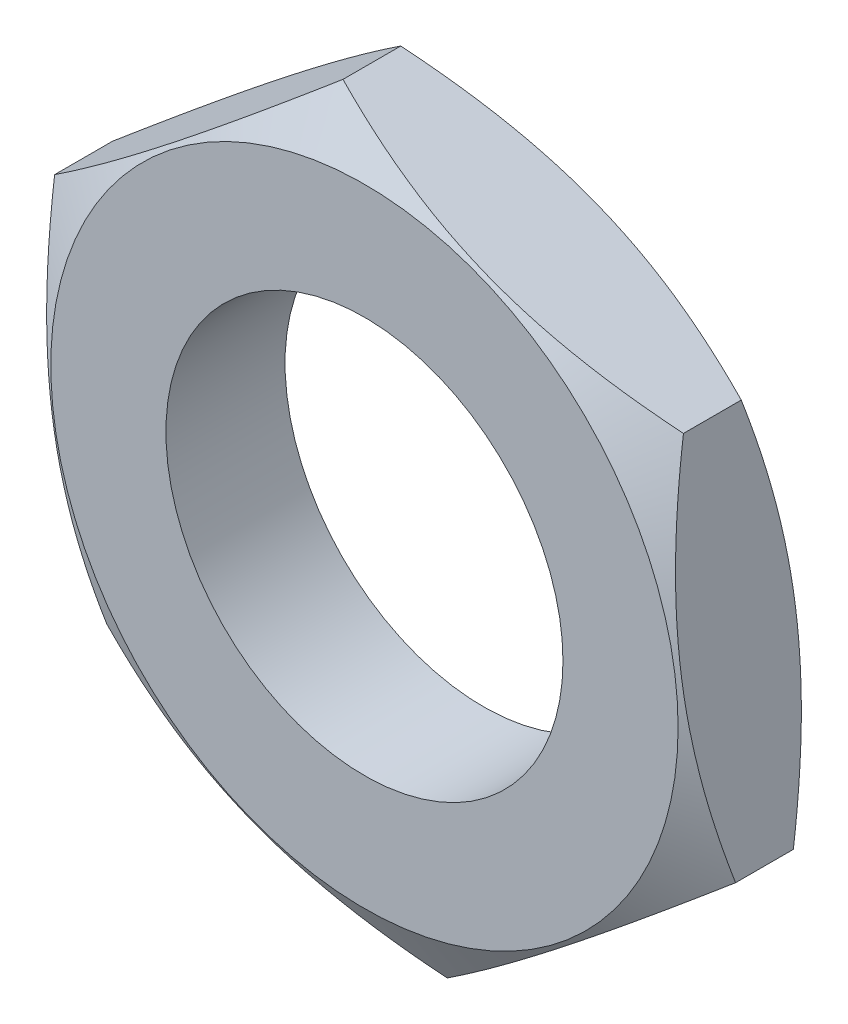
SolidWorks part; units mm, degrees
ref_plane "Front Plane" through (0, 0, 0) normal (0, 0, 1) x (1, 0, 0)
ref_plane "Top Plane" through (0, 0, 0) normal (0, 1, 0) x (1, 0, 0)
ref_plane "Right Plane" through (0, 0, 0) normal (1, 0, 0) x (0, 0, -1)
sketch "Sketch1" plane through (0, 0, 0) normal (0, 0, 1) x (1, 0, 0)
  line L1 (-14.5246, -11.4179) -> (2.6259, -18.2876)
  line L2 (2.6259, -18.2876) -> (17.1505, -6.8697)
  line L3 (17.1505, -6.8697) -> (14.5246, 11.4179)
  line L4 (14.5246, 11.4179) -> (-2.6259, 18.2876)
  line L5 (-2.6259, 18.2876) -> (-17.1505, 6.8697)
  line L6 (-17.1505, 6.8697) -> (-14.5246, -11.4179)
  circle A0 centre (0, 0) radius 10
  circle A1 centre (0, 0) radius 16 construction
  dimension "D1" = 20
  dimension "D2" = 32
extrude "Boss-Extrude1" add sketch "Sketch1" along normal blind 6
sketch "Sketch3" plane through (0, 0, 6) normal (0, 0, 1) x (1, 0, 0)
  circle A0 centre (0, 0) radius 15.8
  dimension "D1" = 31.6
extrude "Cut-Extrude2" cut sketch "Sketch3" against normal blind 10 draft 60 flip side to cut
sketch "Sketch4" plane through (0, 0, 0) normal (0, 0, -1) x (-1, 0, 0)
  circle A0 centre (0, 0) radius 15.8
  dimension "D1" = 31.6
extrude "Cut-Extrude3" cut sketch "Sketch4" against normal blind 5 draft 60 flip side to cut
